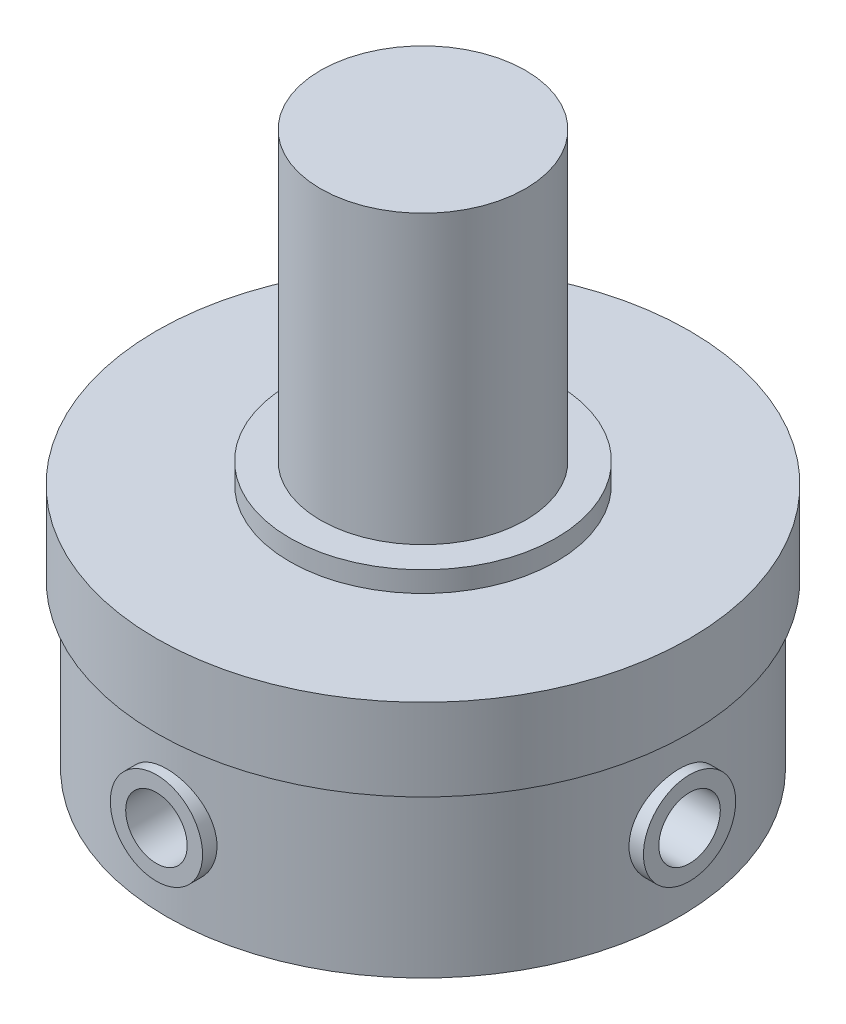
from build123d import *

# Parameters (mm, degrees)
SKETCH1_R           = 125
SKETCH1_R_2         = 100
BOSS_EXTRUDE1_DEPTH = 80
SKETCH2_R           = 130
BOSS_EXTRUDE2_DEPTH = 40
SKETCH3_R           = 50
BOSS_EXTRUDE3_DEPTH = 150
SKETCH4_R           = 65
BOSS_EXTRUDE4_DEPTH = 10
SKETCH5_R           = 15
CUT_EXTRUDE1_DEPTH  = 170
CIRPATTERN1_COUNT   = 4
BOSS_EXTRUDE5_START = -20
SKETCH6_R           = 22.5
SKETCH6_R_2         = 15
BOSS_EXTRUDE5_DEPTH = 25
CIRPATTERN2_COUNT   = 4


with BuildPart() as part:
    # Sketch1 → Boss-Extrude1 (new body)
    with BuildSketch(Plane(origin=(0, 0, 0), x_dir=(1, 0, 0), z_dir=(0, 1, 0))):
        with Locations(Location((0, 0, 0), (0, 0, 270))):
            Circle(SKETCH1_R)
        with Locations(Location((0, 0, 0), (0, 0, 270))):
            Circle(SKETCH1_R_2, mode=Mode.SUBTRACT)
    extrude(amount=BOSS_EXTRUDE1_DEPTH)

    # Sketch2 → Boss-Extrude2 (add)
    with BuildSketch(Plane(origin=(0, 80, 0), x_dir=(1, 0, 0), z_dir=(0, 1, 0))):
        with Locations(Location((0, 0, 0), (0, 0, 270))):
            Circle(SKETCH2_R)
    extrude(amount=BOSS_EXTRUDE2_DEPTH)

    # Sketch3 → Boss-Extrude3 (add)
    with BuildSketch(Plane(origin=(0, 120, 0), x_dir=(1, 0, 0), z_dir=(0, 1, 0))):
        with Locations(Location((0, 0, 0), (0, 0, 270))):
            Circle(SKETCH3_R)
    extrude(amount=BOSS_EXTRUDE3_DEPTH)

    # Sketch4 → Boss-Extrude4 (add)
    with BuildSketch(Plane(origin=(0, 120, 0), x_dir=(1, 0, 0), z_dir=(0, 1, 0))):
        with Locations(Location((0, 0, 0), (0, 0, 270))):
            Circle(SKETCH4_R)
    extrude(amount=BOSS_EXTRUDE4_DEPTH)

    # Sketch5 → Cut-Extrude1 (cut, symmetric)
    with BuildSketch(Plane(origin=(0, 0, 0), x_dir=(0, 0, -1), z_dir=(1, 0, 0))):
        with Locations(Location((0, 40, 0), (0, 0, 180))):
            Circle(SKETCH5_R)
    cut_extrude1 = extrude(amount=CUT_EXTRUDE1_DEPTH, both=True, mode=Mode.SUBTRACT)

    # CirPattern1: Cut-Extrude1 ×4 about axis
    cirpattern1_axis = Axis((0, 80, 0), (0, -1, 0))
    for i in range(1, CIRPATTERN1_COUNT):
        add(cut_extrude1.rotate(cirpattern1_axis, i * 360 / CIRPATTERN1_COUNT), mode=Mode.SUBTRACT)

    # Sketch6 → Boss-Extrude5 (add)
    with BuildSketch(Plane.ZY.offset(125).offset(BOSS_EXTRUDE5_START)):
        with Locations((0, 40)):
            Circle(SKETCH6_R)
        with Locations((0, 40)):
            Circle(SKETCH6_R_2, mode=Mode.SUBTRACT)
    boss_extrude5 = extrude(amount=BOSS_EXTRUDE5_DEPTH)

    # CirPattern2: Boss-Extrude5 ×4 about axis
    cirpattern2_axis = Axis((0, 0, 0), (0, 1, 0))
    for i in range(1, CIRPATTERN2_COUNT):
        add(boss_extrude5.rotate(cirpattern2_axis, i * 360 / CIRPATTERN2_COUNT))


solid = part.part
